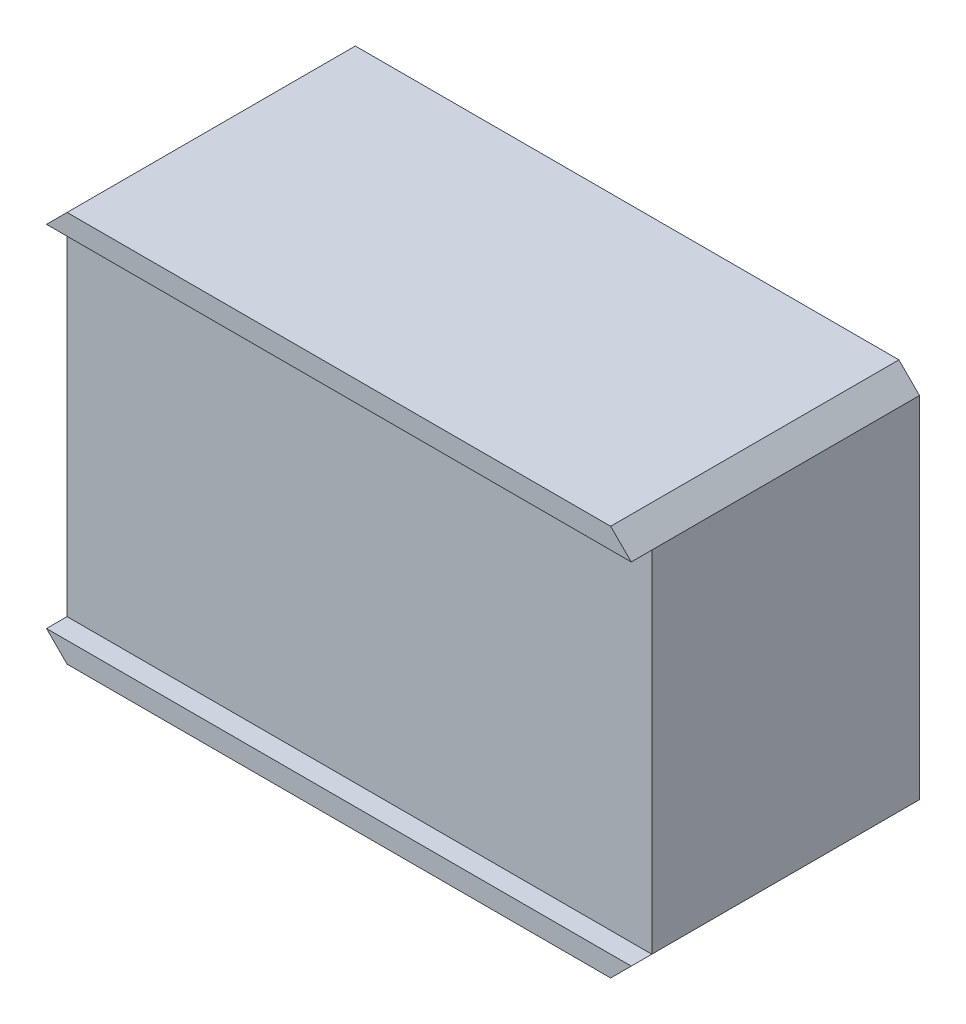
from build123d import *

# Parameters (mm, degrees)
SKETCH_1_W          = 56.8
SKETCH_1_H          = 38
EXTRUDE_1_DEPTH     = 14
CHAMFER_1_SIZE      = 2
SKETCH_2_W          = 2
SKETCH_2_H          = 34
CUT_EXTRUDE_1_DEPTH = 62.508048254


with BuildPart() as part:
    # 草图1 → 凸台-拉伸1 (new, symmetric)
    with BuildSketch(Plane.XY):
        Rectangle(SKETCH_1_W, SKETCH_1_H)
    extrude(amount=EXTRUDE_1_DEPTH, both=True)

    # 倒角1
    chamfer_1_edges = [part.edges().sort_by_distance(p)[0] for p in [
        (28.4, -19, 0),
        (-28.4, -19, 0),
        (-28.4, 19, 0),
        (28.4, 19, 0),
    ]]
    chamfer(chamfer_1_edges, length=CHAMFER_1_SIZE)

    # 草图2 → 切除-拉伸1 (cut, through all)
    with BuildSketch(Plane(origin=(28.4, 0, 0), x_dir=(0, 0, -1), z_dir=(1, 0, 0))):
        with Locations((-13, 0)):
            Rectangle(SKETCH_2_W, SKETCH_2_H)
    extrude(amount=-CUT_EXTRUDE_1_DEPTH, mode=Mode.SUBTRACT)


solid = part.part
